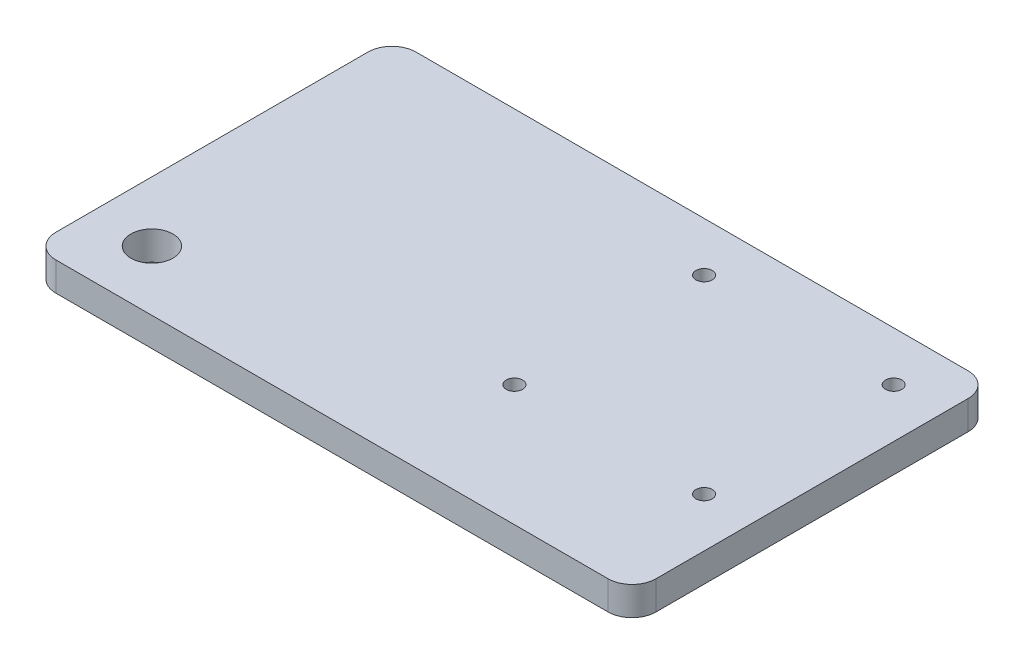
from build123d import *

# Parameters (mm, degrees)
SKETCH_1_W          = 250
SKETCH_1_H          = 150
EXTRUDE_1_DEPTH     = 12
HOLE_WIZARD_M20_1_D = 17.5
HOLE_WIZARD_M8_1_D  = 6.8
FILLET_1_R          = 10


with BuildPart() as part:
    # 草图1 → 凸台-拉伸1 (new body)
    with BuildSketch(Plane(origin=(0, 0, 0), x_dir=(1, 0, 0), z_dir=(0, 1, 0))):
        Rectangle(SKETCH_1_W, SKETCH_1_H)
    extrude(amount=EXTRUDE_1_DEPTH)

    # M20 螺纹孔1 (through all)
    with Locations(Plane(origin=(0, 0, 0), x_dir=(-1, 0, 0), z_dir=(0, -1, 0))):
        with Locations((100, -50)):
            Hole(HOLE_WIZARD_M20_1_D / 2)

    # M8 螺纹孔1 (through all)
    with Locations(Plane(origin=(0, 12, 0), x_dir=(1, 0, 0), z_dir=(0, 1, 0))):
        with Locations((25.5, 54.5), (104.5, 54.5), (25.5, -24.5), (104.5, -24.5)):
            Hole(HOLE_WIZARD_M8_1_D / 2)

    # 圆角1
    fillet_1_edges = [part.edges().sort_by_distance(p)[0] for p in [
        (125, 6, 75),
        (-125, 6, 75),
        (-125, 6, -75),
        (125, 6, -75),
    ]]
    fillet(fillet_1_edges, radius=FILLET_1_R)


solid = part.part
